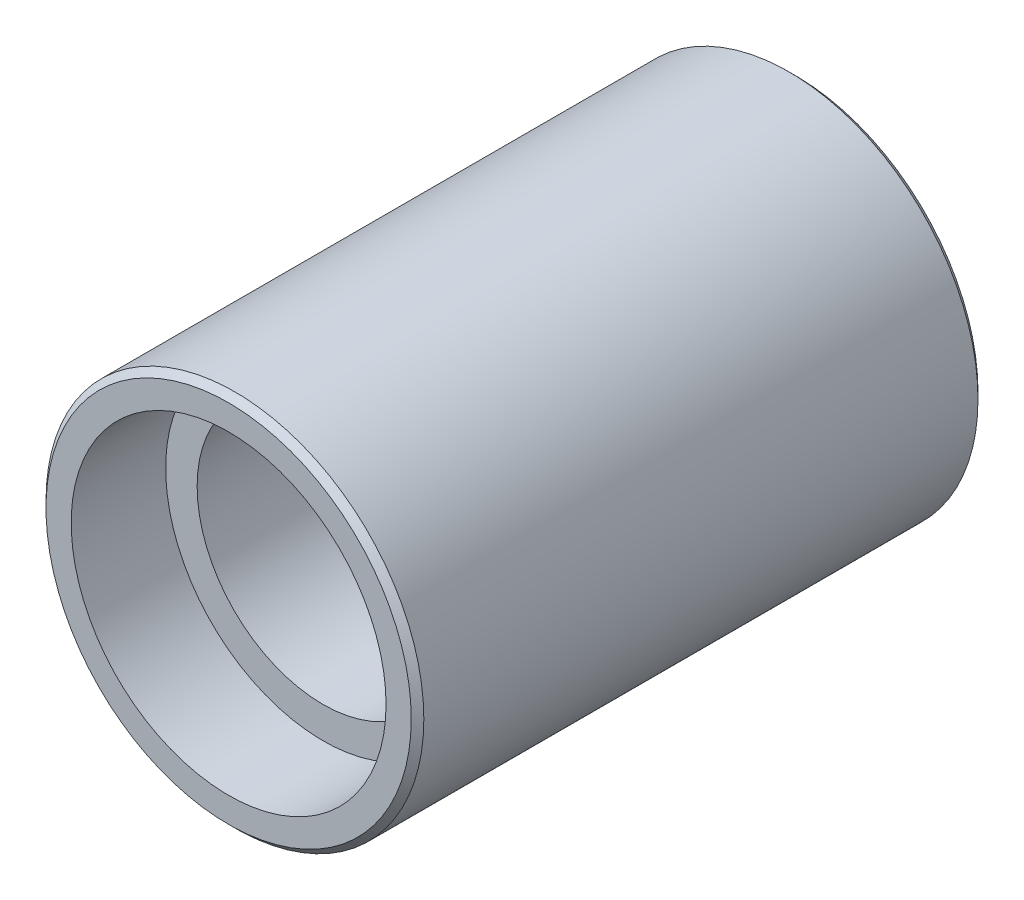
from build123d import *

# Parameters (mm, degrees)
SKETCH1_R           = 6
SKETCH1_R_2         = 4
BOSS_EXTRUDE1_DEPTH = 9
SKETCH2_R           = 5
CUT_EXTRUDE1_DEPTH  = 3
CHAMFER1_SIZE       = 0.2


with BuildPart() as part:
    # Sketch1 → Boss-Extrude1 (new, symmetric)
    with BuildSketch(Plane.XY):
        Circle(SKETCH1_R)
        Circle(SKETCH1_R_2, mode=Mode.SUBTRACT)
    extrude(amount=BOSS_EXTRUDE1_DEPTH, both=True)

    # Sketch2 → Cut-Extrude1 (cut)
    with BuildSketch(Plane.XY.offset(9)):
        Circle(SKETCH2_R)
    cut_extrude1 = extrude(amount=-CUT_EXTRUDE1_DEPTH, mode=Mode.SUBTRACT)

    # Mirror1: Cut-Extrude1 across plane
    add(cut_extrude1.mirror(Plane.XY), mode=Mode.SUBTRACT)

    # Chamfer1
    chamfer1_edges = [part.edges().sort_by_distance(p)[0] for p in [
        (-6, 0, -9),
        (-6, 0, 9),
    ]]
    chamfer(chamfer1_edges, length=CHAMFER1_SIZE)


solid = part.part
